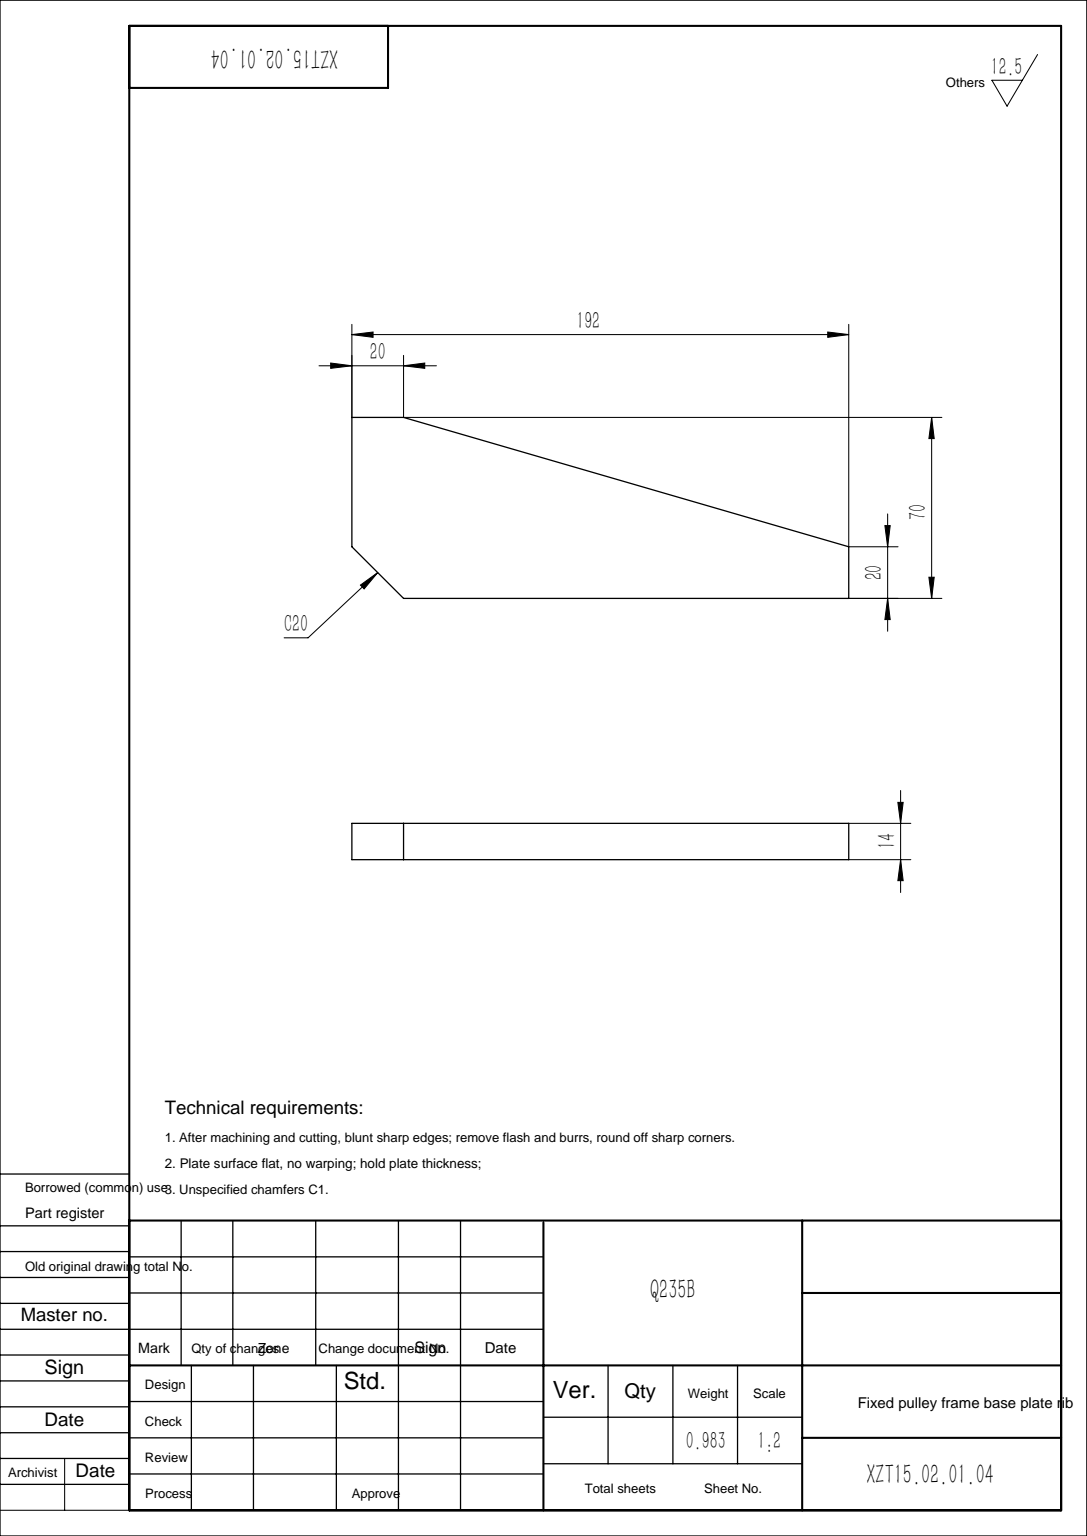
from build123d import *

# Parameters (mm, degrees)
BOSS_EXTRUDE1_DEPTH = 7
CHAMFER1_SIZE       = 20


with BuildPart() as part:
    # Sketch1 → Boss-Extrude1 (new, symmetric)
    with BuildSketch(Plane.XY):
        Polygon((0, 0), (192, 0), (192, 20), (20, 70), (0, 70), align=None)
    extrude(amount=BOSS_EXTRUDE1_DEPTH, both=True)

    # Chamfer1
    chamfer1_edges = [part.edges().sort_by_distance(p)[0] for p in [
        (0, 0, 0),
    ]]
    chamfer(chamfer1_edges, length=CHAMFER1_SIZE)


solid = part.part
